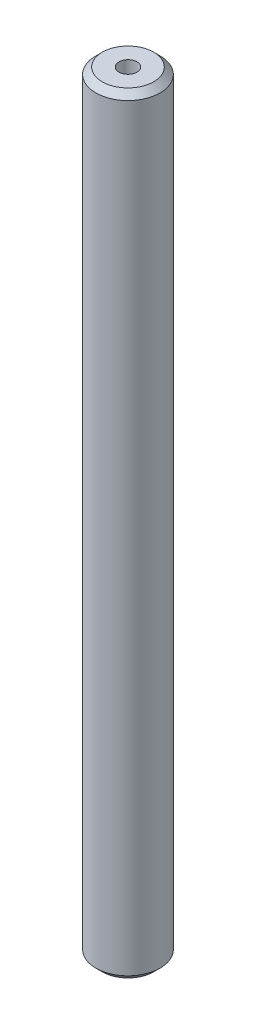
SolidWorks part; units mm, degrees
ref_plane "Front Plane" through (0, 0, 0) normal (0, 0, 1) x (1, 0, 0)
ref_plane "Top Plane" through (0, 0, 0) normal (0, 1, 0) x (1, 0, 0)
ref_plane "Right Plane" through (0, 0, 0) normal (1, 0, 0) x (0, 0, -1)
sketch "Sketch1" plane through (0, 0, 0) normal (0, 1, 0) x (1, 0, 0)
  circle A0 centre (0, 0) radius 25
  dimension "D1" = 50
extrude "Boss-Extrude1" add sketch "Sketch1" along normal blind 600
chamfer "Chamfer1" distance 5 angle 45 2 edges at (0, 0, 25) (0, 600, 25)
hole_wizard "M16 Tapped Hole1" positions "Sketch2" profile "Sketch3" tap size "M16" standard "ISO"
sketch "Sketch2" plane through (0, 600, 0) normal (0, 1, 0) x (1, 0, 0)
  point P0 (0, 0)
sketch "Sketch3" plane through (0, 600, 0) normal (1, 0, 0) x (0, 0, 1)
  line L0 (0, 0) -> (0, 42.206)
  line L1 (0, 42.206) -> (7, 38)
  line L2 (7, 38) -> (7, 0)
  line L5 (7, 0) -> (0, 0)
  line L10 (0, 42.206) -> (-7, 38) construction
  line L11 (0, -6.35) -> (0, 107.95) construction
  dimension "螺纹孔钻头直径" = 14
  dimension "螺纹孔钻头深度" = 38
  dimension "导头角度" = 118
cosmetic thread "Cosmetic Thread1"
hole_wizard "M16 Tapped Hole2" positions "Sketch4" profile "Sketch5" tap size "M16" standard "ISO"
sketch "Sketch4" plane through (0, 0, 0) normal (0, -1, 0) x (-1, 0, 0)
  point P0 (0, 0)
sketch "Sketch5" plane through (0, 0, 0) normal (1, 0, 0) x (0, 0, -1)
  line L0 (0, 0) -> (0, 42.206)
  line L1 (0, 42.206) -> (7, 38)
  line L2 (7, 38) -> (7, 0)
  line L5 (7, 0) -> (0, 0)
  line L10 (0, 42.206) -> (-7, 38) construction
  line L11 (0, -6.35) -> (0, 107.95) construction
  dimension "螺纹孔钻头直径" = 14
  dimension "螺纹孔钻头深度" = 38
  dimension "导头角度" = 118
cosmetic thread "Cosmetic Thread2"
